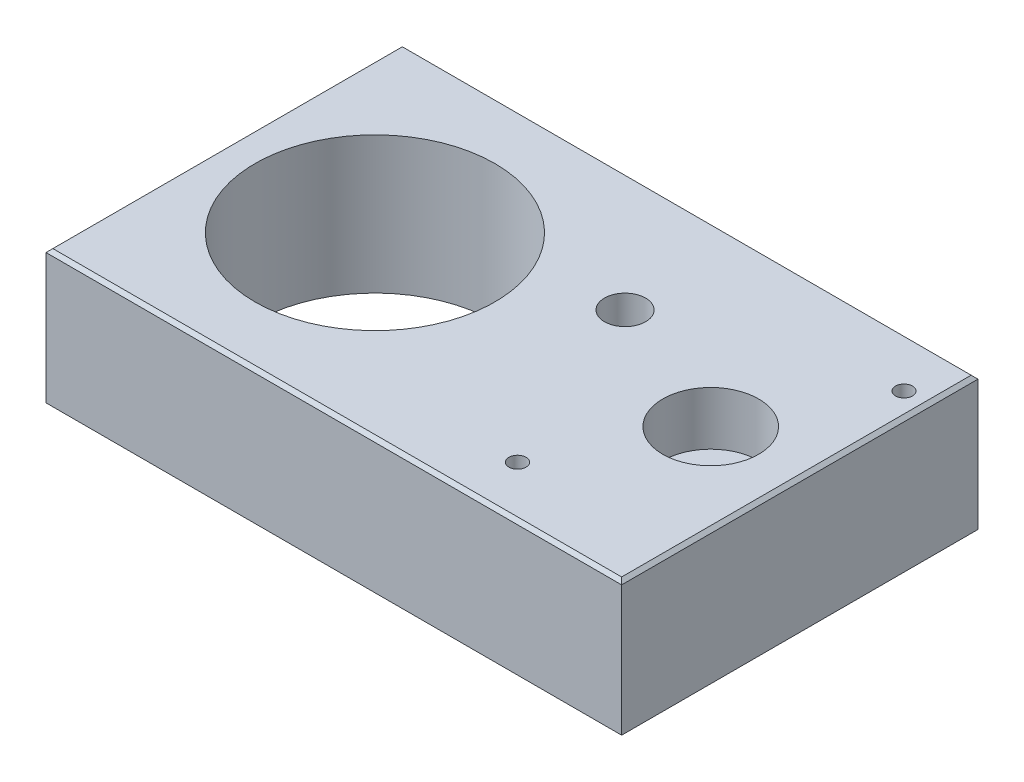
from build123d import *

# Parameters (mm, degrees)
SKETCH1_W           = 84
SKETCH1_H           = 52
BOSS_EXTRUDE1_DEPTH = 20
SKETCH2_R           = 17.5
CUT_EXTRUDE1_DEPTH  = 20
SKETCH3_R           = 3
CUT_EXTRUDE2_DEPTH  = 20
SKETCH4_R           = 1.25
CUT_EXTRUDE3_DEPTH  = 20
SKETCH5_R           = 4
CUT_EXTRUDE4_DEPTH  = 20
SKETCH6_R           = 7
CUT_EXTRUDE5_DEPTH  = 7.8
CHAMFER1_SIZE       = 0.5


with BuildPart() as part:
    # Sketch1 → Boss-Extrude1 (new body)
    with BuildSketch(Plane(origin=(0, 0, 0), x_dir=(1, 0, 0), z_dir=(0, 1, 0))):
        Rectangle(SKETCH1_W, SKETCH1_H)
    extrude(amount=BOSS_EXTRUDE1_DEPTH)

    # Sketch2 → Cut-Extrude1 (cut)
    with BuildSketch(Plane(origin=(0, 20, 0), x_dir=(1, 0, 0), z_dir=(0, 1, 0))):
        with Locations(Location((-20, 0, 0), (0, 0, 270))):
            Circle(SKETCH2_R)
    extrude(amount=-CUT_EXTRUDE1_DEPTH, mode=Mode.SUBTRACT)

    # Sketch3 → Cut-Extrude2 (cut)
    with BuildSketch(Plane(origin=(0, 20, 0), x_dir=(1, 0, 0), z_dir=(0, 1, 0))):
        with Locations(Location((8, 8.5, 0), (0, 0, 270))):
            Circle(SKETCH3_R)
    extrude(amount=-CUT_EXTRUDE2_DEPTH, mode=Mode.SUBTRACT)

    # Sketch4 → Cut-Extrude3 (cut)
    with BuildSketch(Plane(origin=(0, 20, 0), x_dir=(1, 0, 0), z_dir=(0, 1, 0))):
        with Locations(Location((19.4, -18.6, 0), (0, 0, 270))):
            Circle(SKETCH4_R)
        with Locations(Location((38.6, 18.6, 0), (0, 0, 270))):
            Circle(SKETCH4_R)
    extrude(amount=-CUT_EXTRUDE3_DEPTH, mode=Mode.SUBTRACT)

    # Sketch5 → Cut-Extrude4 (cut)
    with BuildSketch(Plane(origin=(0, 20, 0), x_dir=(1, 0, 0), z_dir=(0, 1, 0))):
        with Locations(Location((29, 0, 0), (0, 0, 270))):
            Circle(SKETCH5_R)
    extrude(amount=-CUT_EXTRUDE4_DEPTH, mode=Mode.SUBTRACT)

    # Sketch6 → Cut-Extrude5 (cut)
    with BuildSketch(Plane(origin=(0, 20, 0), x_dir=(1, 0, 0), z_dir=(0, 1, 0))):
        with Locations(Location((29, 0, 0), (0, 0, 270))):
            Circle(SKETCH6_R)
    extrude(amount=-CUT_EXTRUDE5_DEPTH, mode=Mode.SUBTRACT)

    # Chamfer1
    chamfer1_edges = [part.edges().sort_by_distance(p)[0] for p in [
        (-42, 20, 0),
        (0, 20, 26),
        (42, 20, 0),
        (0, 0, 26),
        (-42, 0, 0),
        (0, 0, -26),
        (42, 0, 0),
        (0, 20, -26),
    ]]
    chamfer(chamfer1_edges, length=CHAMFER1_SIZE)


solid = part.part
